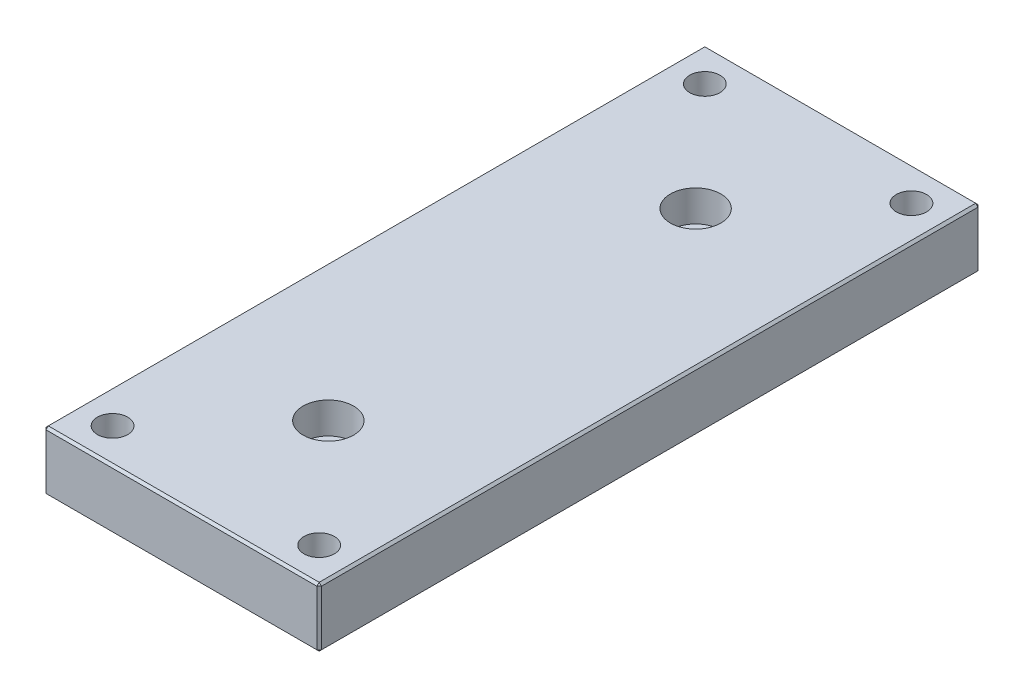
SolidWorks part; units mm, degrees
material "Al6061"
ref_plane "Front" through (0, 0, 0) normal (0, 0, 1) x (1, 0, 0)
ref_plane "Top" through (0, 0, 0) normal (0, 1, 0) x (1, 0, 0)
ref_plane "Right" through (0, 0, 0) normal (1, 0, 0) x (0, 0, -1)
sketch "草图1" plane through (0, 0, 0) normal (0, 0, 1) x (1, 0, 0)
  line L1 (-30, 6.5) -> (30, 6.5)
  line L2 (-30, 6.5) -> (-30, -6.5)
  line L3 (-30, -6.5) -> (30, -6.5)
  line L4 (30, 6.5) -> (30, -6.5)
  line L5 (-30, 6.5) -> (30, -6.5) construction
  line L6 (-30, -6.5) -> (30, 6.5) construction
  point P0 (0, 0)
  dimension "D1" = 13
  dimension "D2" = 60
extrude "凸台-拉伸1" add sketch "草图1" along normal blind 144
hole_wizard "打孔尺寸根据内六角圆柱头螺钉的类型2" positions "草图7" profile "草图6" counterbore size "M6" standard "Gb" end condition through all
sketch "草图7" plane through (0, 6.5, 0) normal (0, 1, 0) x (1, 0, 0)
  line L0 (0, 0) -> (0, -144) construction
  line L1 (30, -144) -> (-30, -144) construction
  line L3 (30, -72) -> (-30, -72) construction
  line L4 (30, -144) -> (30, 0) construction
  line L5 (-30, -144) -> (-30, 0) construction
  point P4 (0, -32)
  point P6 (0, -112)
  dimension "D1" = 80
sketch "草图6" plane through (0, 6.5, 32) normal (1, 0, 0) x (0, 0, 1)
  line L0 (0, 0) -> (0, 13)
  line L1 (0, 13) -> (3.3, 13)
  line L3 (3.3, 13) -> (3.3, 6.8)
  line L4 (3.3, 6.8) -> (5.5, 6.8)
  line L5 (5.5, 6.8) -> (5.5, 0)
  line L7 (5.5, 0) -> (0, 0)
  line L11 (0, -6.35) -> (0, 107.95) construction
  dimension "通孔孔直径" = 6.6
  dimension "通孔孔深度" = 13
  dimension "柱形沉头孔直径" = 11
  dimension "柱形沉头孔深度" = 6.8
chamfer "倒角1" distance 0.5 angle 45 12 edges at (0, -6.5, 144) (0, 6.5, 144) (-30, 6.5, 72) (-30, 0, 144) (-30, -6.5, 72) (-30, 0, 0) (30, -6.5, 72) (30, 0, 144) (30, 6.5, 72) (0, -6.5, 0) (30, 0, 0) (0, 6.5, 0)
hole_wizard "打孔尺寸根据内六角圆柱头螺钉的类型2" positions "草图9" profile "草图8" counterbore size "M6" standard "Gb" end condition through all
sketch "草图9" plane through (0, -6.5, 0) normal (0, -1, 0) x (-1, 0, 0)
  line L0 (29.5, -72) -> (-84.9875, -72) construction
  line L1 (29.5, -143.5) -> (29.5, -0.5) construction
  line L3 (0, -143.5) -> (0, -0.5) construction
  line L4 (-29.5, -143.5) -> (29.5, -143.5) construction
  line L5 (29.5, -0.5) -> (-29.5, -0.5) construction
  point P0 (-22.5, -136.5)
  point P2 (22.5, -136.5)
  point P4 (-22.5, -7.5)
  point P6 (22.5, -7.5)
  dimension "D1" = 45
  dimension "D2" = 129
sketch "草图8" plane through (22.5, -6.5, 136.5) normal (1, 0, 0) x (0, 0, -1)
  line L0 (0, 0) -> (0, 13)
  line L1 (0, 13) -> (3.3, 13)
  line L3 (3.3, 13) -> (3.3, 6.8)
  line L4 (3.3, 6.8) -> (5.5, 6.8)
  line L5 (5.5, 6.8) -> (5.5, 0)
  line L7 (5.5, 0) -> (0, 0)
  line L11 (0, -6.35) -> (0, 107.95) construction
  dimension "通孔孔直径" = 6.6
  dimension "通孔孔深度" = 13
  dimension "柱形沉头孔直径" = 11
  dimension "柱形沉头孔深度" = 6.8
